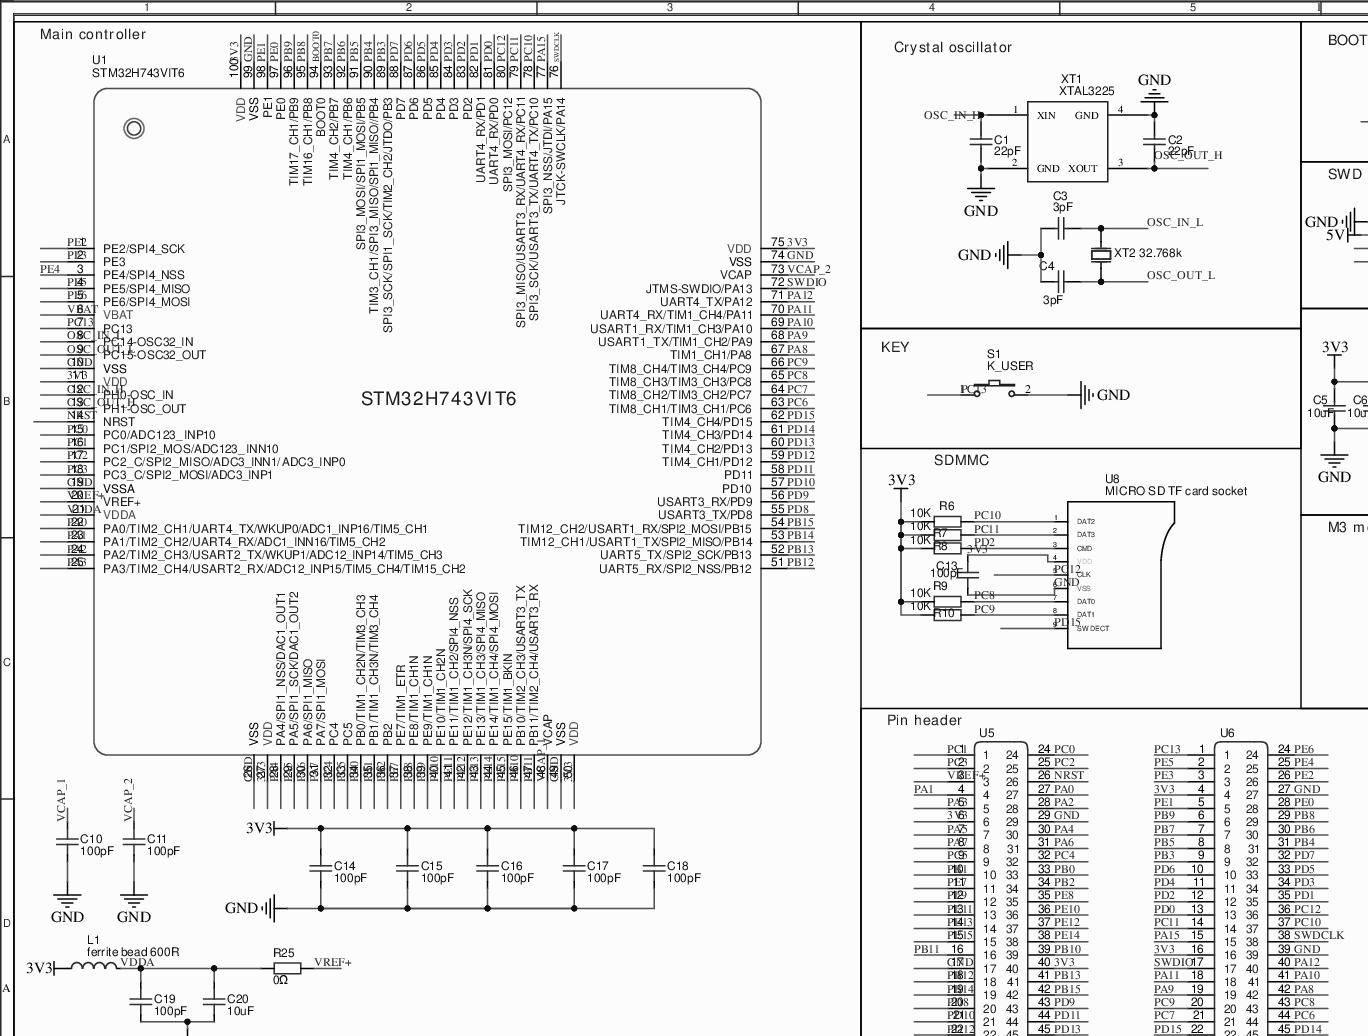
[diagram p0: MISC51975-3.schdoc, top left]
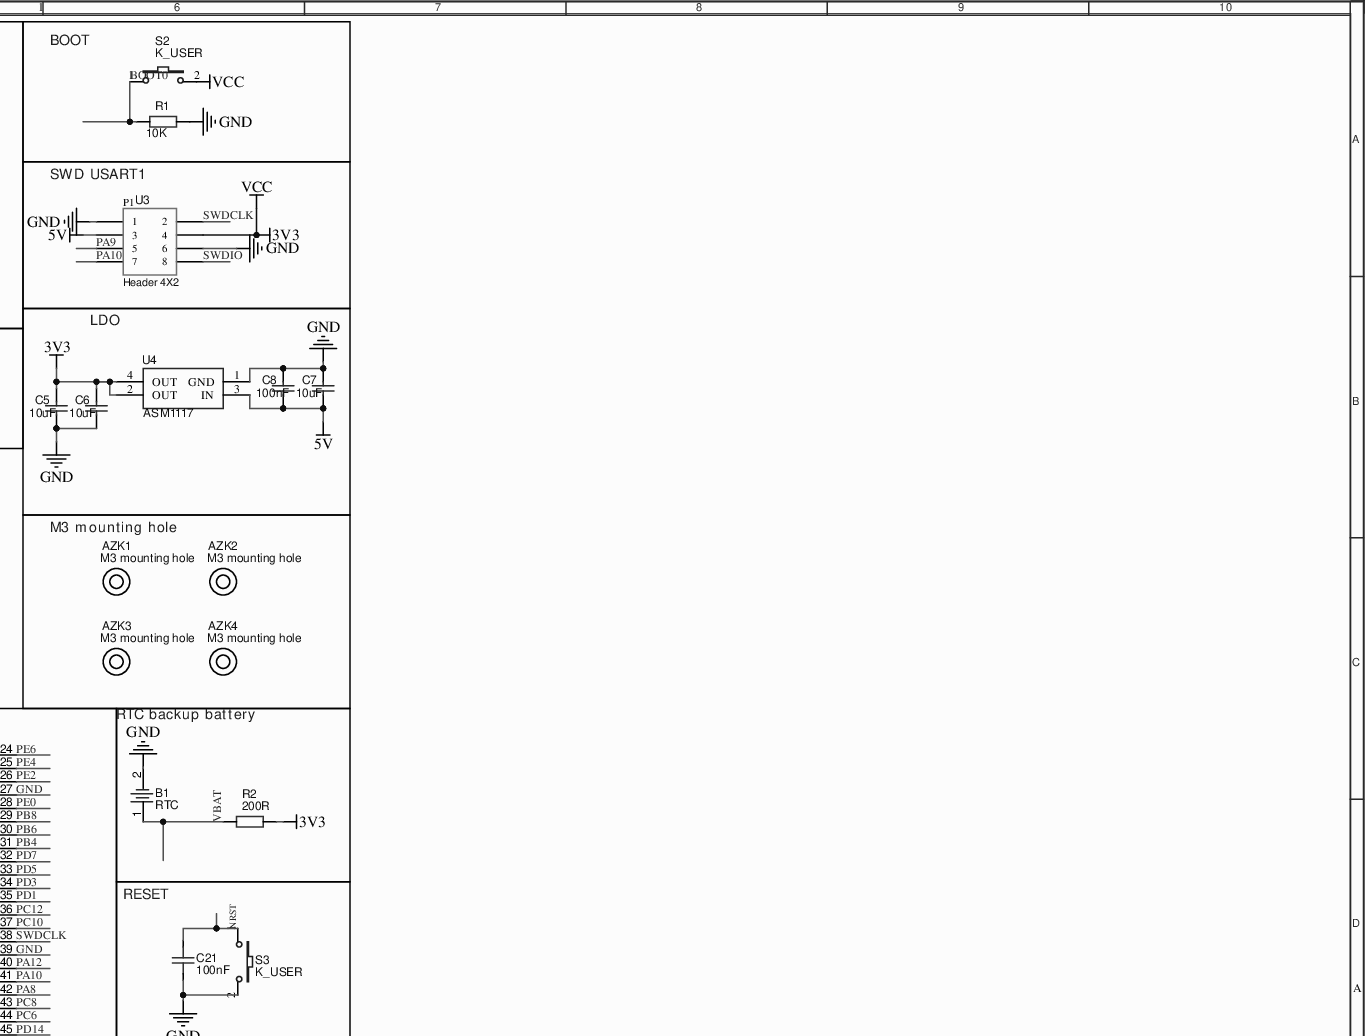
[diagram p1: MISC51975-3.schdoc, top right]
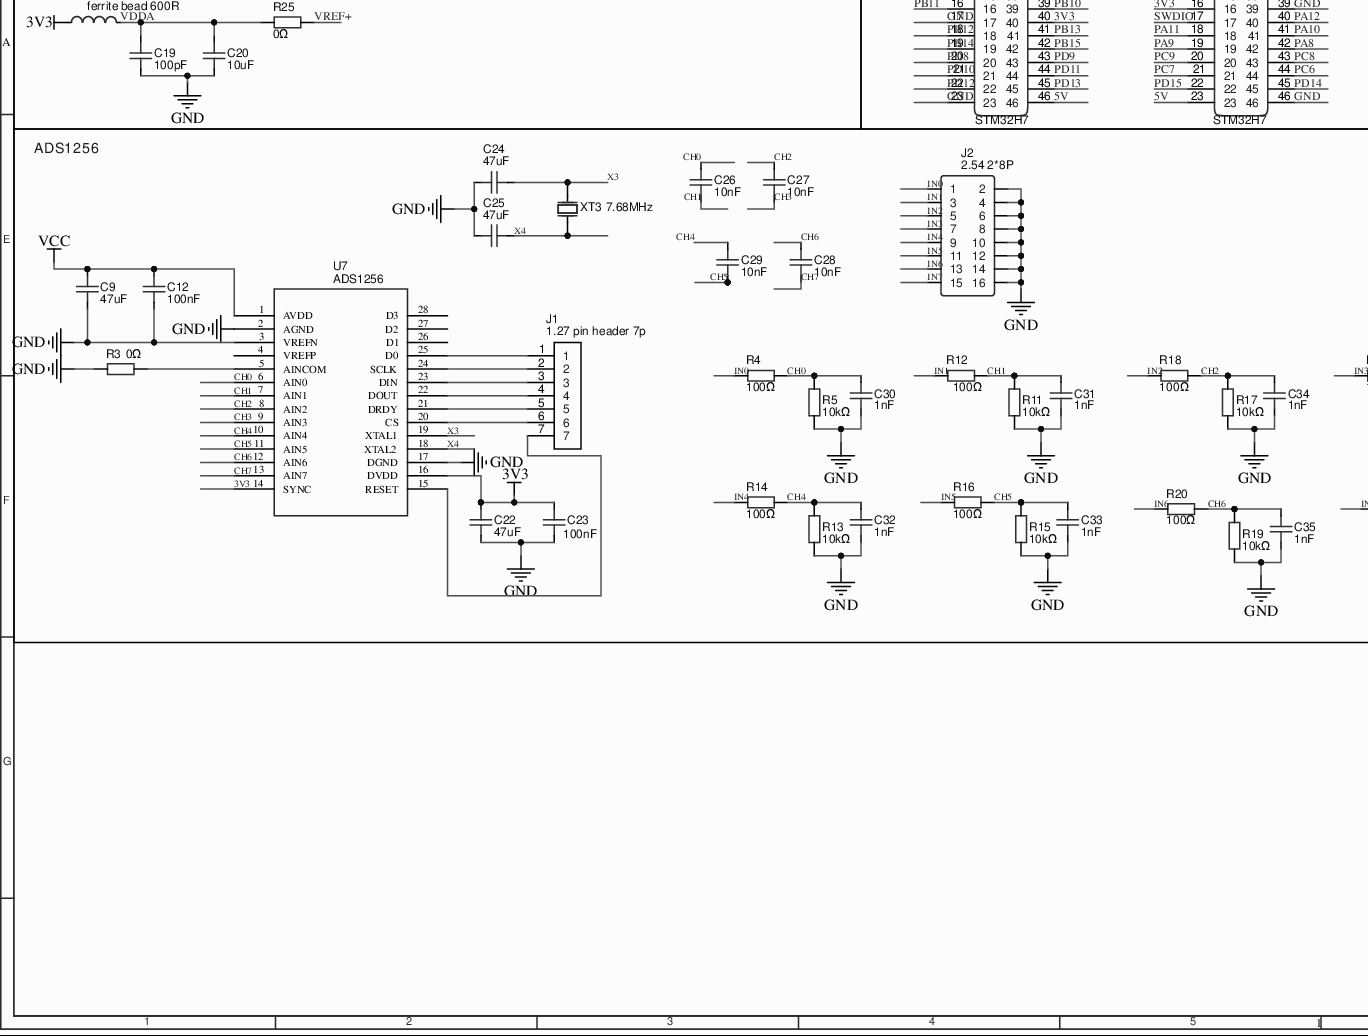
[diagram p2: MISC51975-3.schdoc, bottom left]
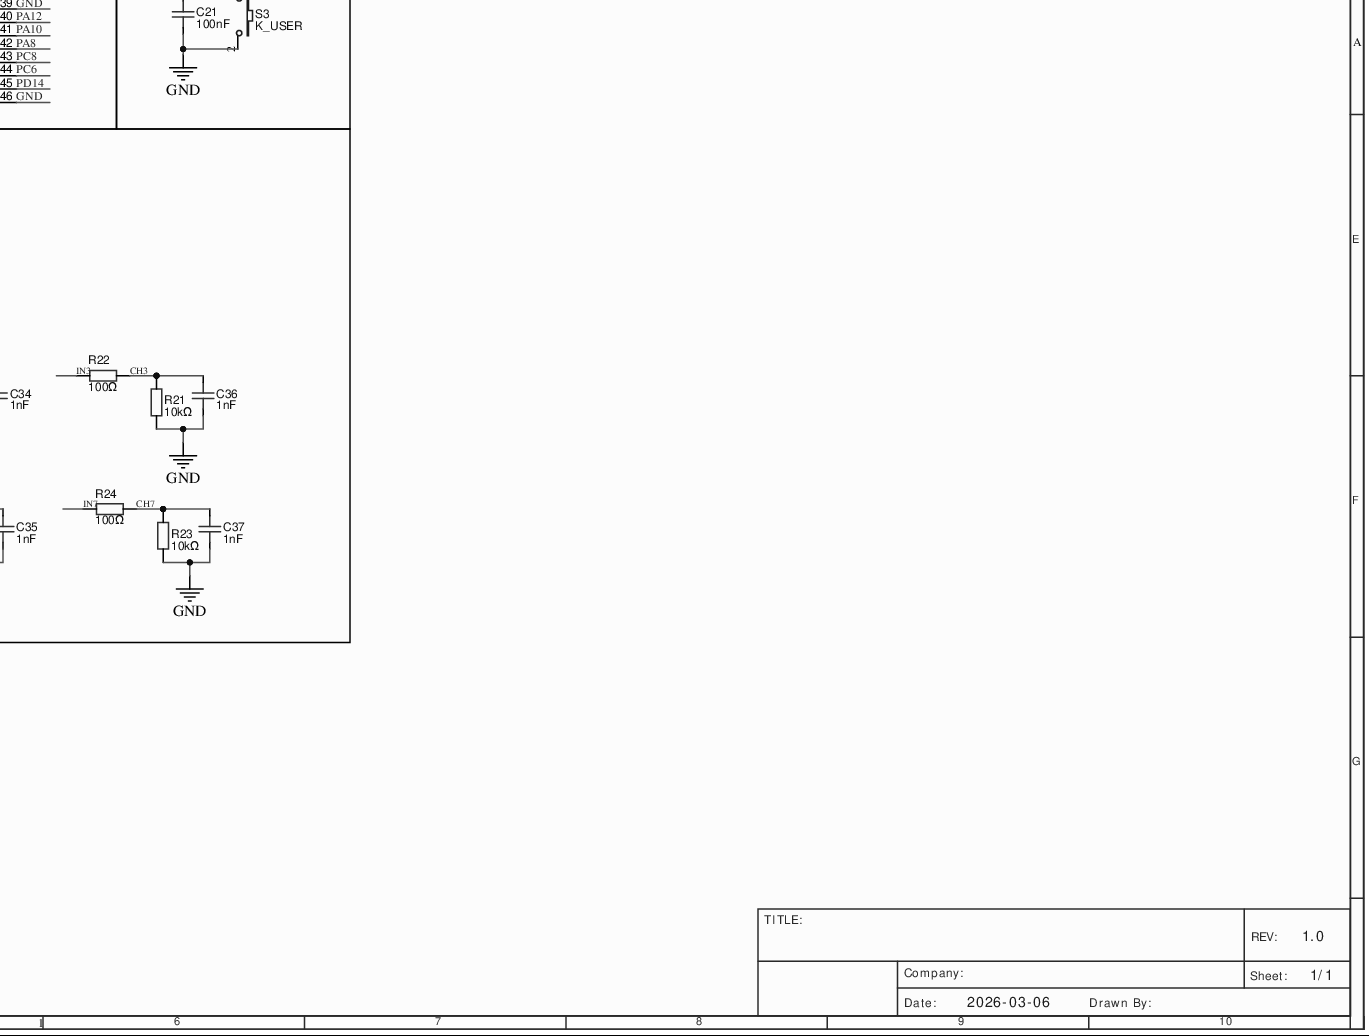
[diagram p3: MISC51975-3.schdoc, bottom right]
# Altium project MISC51975-2.PrjPcb
1 sheet, 83 parts. Net scope: global (net labels, ports and power ports of the same name join across sheets).
Board file: MISC51975.pcbdoc

## Sheet MISC51975-3.schdoc
size 503 x 376 mm; Name: MISC51975; @Project Name: MISC51975; REV: 1.0; Date: 2026-03-06; Sheet: 1/1; Manufacturer Part: ?

### Parts
AZK1  M3 mounting hole  [M3安装孔(非金属化)]
AZK2  M3 mounting hole  [M3安装孔(非金属化)]
AZK3  M3 mounting hole  [M3安装孔(非金属化)]
AZK4  M3 mounting hole  [M3安装孔(非金属化)]
B1  RTC  [焊盘引出RTC]
C1  22pF  [C0402]
C2  22pF  [C0402]
C3  3pF  [C0402]
C4  3pF  [C0402]
C5  10uF  [C0402]
C6  10uF  [C0402]
C7  10uF  [C0402]
C8  100nF  [C0402]
C9  47uF  [C0402]
C10  100pF  [C0402]
C11  100pF  [C0402]
C12  100nF  [C0402]
C13  100pF  [C0402]
C14  100pF  [C0402]
C15  100pF  [C0402]
C16  100pF  [C0402]
C17  100pF  [C0402]
C18  100pF  [C0402]
C19  100pF  [C0402]
C20  10uF  [C0402]
C21  100nF  [C0402]
C22  47uF  [C0402]
C23  100nF  [C0402]
C24  47uF  [C0402]
C25  47uF  [C0402]
C26  10nF  [C0402]
C27  10nF  [C0402]
C28  10nF  [C0402]
C29  10nF  [C0402]
C30  1nF  [C0402]
C31  1nF  [C0402]
C32  1nF  [C0402]
C33  1nF  [C0402]
C34  1nF  [C0402]
C35  1nF  [C0402]
C36  1nF  [C0402]
C37  1nF  [C0402]
J1  1.27 pin header 7p  [1.27排针7P]
J2  2.54 2*8P  [HDR-TH_16P-P2.54-V-R2-C8-S2.54]
L1  ferrite bead 600R  [L0402]
R1  10K  [贴片电阻0402封装]
R2  200R  [贴片电阻0402封装]
R3  0Ω  [贴片电阻0402封装]
R4  100Ω  [贴片电阻0402封装]
R5  10kΩ  [贴片电阻0402封装]
R6  10K  [贴片电阻0402封装]
R7  10K  [贴片电阻0402封装]
R8  10K  [贴片电阻0402封装]
R9  10K  [贴片电阻0402封装]
R10  10K  [贴片电阻0402封装]
R11  10kΩ  [贴片电阻0402封装]
R12  100Ω  [贴片电阻0402封装]
R13  10kΩ  [贴片电阻0402封装]
R14  100Ω  [贴片电阻0402封装]
R15  10kΩ  [贴片电阻0402封装]
R16  100Ω  [贴片电阻0402封装]
R17  10kΩ  [贴片电阻0402封装]
R18  100Ω  [贴片电阻0402封装]
R19  10kΩ  [贴片电阻0402封装]
R20  100Ω  [贴片电阻0402封装]
R21  10kΩ  [贴片电阻0402封装]
R22  100Ω  [贴片电阻0402封装]
R23  10kΩ  [贴片电阻0402封装]
R24  100Ω  [贴片电阻0402封装]
R25  0Ω  [贴片电阻0402封装]
S1  K_USER  [按键开关4.5]
S2  K_USER  [按键开关4.5]
S3  K_USER  [按键开关4.5]
U1  STM32H743VIT6  [STM32H743VIT6]
U3  HDR_2*4P  [HDR_2*4P]  (value not drawn)
U4  ASM1117  [AMS1117-SOT-223]
U5  STM32H7  [2*23]
U6  STM32H7  [2*23]
U7  ADS1256  [SSOP-28_L10.2-W5.3-P0.65-LS7.8-BL]
U8  MICRO SD TF card socket  [MICRO SD TF卡座]
XT1  XTAL3225  [XTAL3225]
XT2  32.768k  [SMD-2012_2P]
XT3  7.68MHz  [SMD-2012_2P]

### Blocks framed on the sheet
Main controller: C10 C11 C14-C20 L1 R25 U1
Crystal oscillator: C1-C4 XT1 XT2
BOOT: R1 S2
SWD USART1: U3
KEY: S1
LDO: C5-C8 U4
M3 mounting hole: AZK1-AZK4
Pin header: U5 U6
RTC backup battery: B1 R2
RESET: C21 S3
ADS1256: C9 C12 C22-C37 J1 J2 R3-R5 R11-R24 U7 XT3

### Nets
3V3: C5.2 C6.2 C9.2 C12.2 C13.2 C14.2 C15.2 C16.2 C17.2 C18.2 C22.2 C23.2 L1.1 R2.1 R6.1 R7.1 R8.1 R9.1 R10.1 S2.2 U1.11(VDD) U1.27(VDD) U1.50(VDD) U1.75(VDD) U1.100(VDD) U3.4 U4.2(OUT) U4.4(OUT) U5.6 U5.40 U6.4 U6.16 U7.1(AVDD) U7.14(SYNC) U7.16(DVDD) U8.4(VDD)  [also labelled VCC]
5V: C7.1 C8.1 U3.3 U4.3(IN) U5.46 U6.23
GND: B1.2 C1.1 C2.2 C3.2 C4.2 C5.1 C6.1 C7.2 C8.2 C9.1 C10.1 C11.1 C12.1 C13.1 C14.1 C15.1 C16.1 C17.1 C18.1 C19.1 C20.1 C21.1 C22.1 C23.1 C24.2 C25.2 C30.2 C31.2 C32.2 C33.2 C34.2 C35.2 C36.2 C37.2 J2.2 J2.4 J2.6 J2.8 J2.10 J2.12 J2.14 J2.16 R1.2 R3.1 R5.1 R11.1 R13.1 R15.1 R17.1 R19.1 R21.1 R23.1 S1.2 S3.2 U1.10(VSS) U1.19(VSSA) U1.26(VSS) U1.49(VSS) U1.74(VSS) U1.99(VSS) U3.1 U3.6 U4.1(GND) U5.17 U5.23 U5.29 U6.27 U6.39 U6.46 U7.2(AGND) U7.3(VREFN) U7.17(DGND) U8.6(VSS) XT1.2(GND) XT1.4(GND)
BOOT0: R1.1 S2.1 U1.94(BOOT0)
CH0: C26.1 C30.1 R4.2 R5.2 U7.6(AIN0)
CH1: C26.2 C31.1 R11.2 R12.2 U7.7(AIN1)
CH2: C27.1 C34.1 R17.2 R18.2 U7.8(AIN2)
CH3: C27.2 C36.1 R21.2 R22.2 U7.9(AIN3)
CH4: C29.1 C32.1 R13.2 R14.2 U7.10(AIN4)
CH5: C29.2 C33.1 R15.2 R16.2 U7.11(AIN5)
CH6: C28.1 C35.1 R19.2 R20.2 U7.12(AIN6)
CH7: C28.2 C37.1 R23.2 R24.2 U7.13(AIN7)
IN0: J2.1 R4.1
IN1: J2.3 R12.1
IN2: J2.5 R18.1
IN3: J2.7 R22.1
IN4: J2.9 R14.1
IN5: J2.11 R16.1
IN6: J2.13 R20.1
IN7: J2.15 R24.1
NRST: C21.2 S3.1 U1.14(NRST) U5.26
OSC_IN_H: C1.2 U1.12(PH0-OSC_IN) XT1.1(XIN)
OSC_IN_L: C3.1 U1.8(PC14-OSC32_IN) XT2.1(OSC1)
OSC_OUT_H: C2.1 U1.13(PH1-OSC_OUT) XT1.3(XOUT)
OSC_OUT_L: C4.1 U1.9(PC15-OSC32_OUT) XT2.2(OSC2)
PA0: U1.22(PA0/TIM2_CH1/UART4_TX/WKUP0/ADC1_INP16/TIM5_CH1) U5.27
PA1: U1.23(PA1/TIM2_CH2/UART4_RX/ADC1_INN16/TIM5_CH2) U5.4
PA2: U1.24(PA2/TIM2_CH3/USART2_TX/WKUP1/ADC12_INP14/TIM5_CH3) U5.28
PA3: U1.25(PA3/TIM2_CH4/USART2_RX/ADC12_INP15/TIM5_CH4/TIM15_CH2) U5.5
PA4: U1.28(PA4/SPI1_NSS/DAC1_OUT1) U5.30
PA5: U1.29(PA5/SPI1_SCK/DAC1_OUT2) U5.7
PA6: U1.30(PA6/SPI1_MISO) U5.31
PA7: U1.31(PA7/SPI1_MOSI) U5.8
PA8: U1.67(TIM1_CH1/PA8) U6.42
PA9: U1.68(USART1_TX/TIM1_CH2/PA9) U3.5 U6.19
PA10: U1.69(USART1_RX/TIM1_CH3/PA10) U3.7 U6.41
PA11: U1.70(UART4_RX/TIM1_CH4/PA11) U6.18
PA12: U1.71(UART4_TX/PA12) U6.40
PA15: U1.77(SPI3_NSS/JTDI/PA15) U6.15
PB0: U1.34(PB0/TIM1_CH2N/TIM3_CH3) U5.33
PB1: U1.35(PB1/TIM1_CH3N/TIM3_CH4) U5.10
PB2: U1.36(PB2) U5.34
PB3: U1.89(SPI3_SCK/SPI1_SCK/TIM2_CH2/JTDO/PB3) U6.9
PB4: U1.90(TIM3_CH1/SPI3_MISO/SPI1_MISO//PB4) U6.31
PB5: U1.91(SPI3_MOSI/SPI1_MOSI/PB5) U6.8
PB6: U1.92(TIM4_CH1/PB6) U6.30
PB7: U1.93(TIM4_CH2/PB7) U6.7
PB8: U1.95(TIM16_CH1/PB8) U6.29
PB9: U1.96(TIM17_CH1/PB9) U6.6
PB10: U1.46(PB10/TIM2_CH3/USART3_TX) U5.39
PB11: U1.47(PB11/TIM2_CH4/USART3_RX) U5.16
PB12: U1.51(UART5_RX/SPI2_NSS/PB12) U5.18
PB13: U1.52(UART5_TX/SPI2_SCK/PB13) U5.41
PB14: U1.53(TIM12_CH1/USART1_TX/SPI2_MISO/PB14) U5.19
PB15: U1.54(TIM12_CH2/USART1_RX/SPI2_MOSI/PB15) U5.42
PC0: U1.15(PC0/ADC123__INP10) U5.24
PC1: U1.16(PC1/SPI2_MOS/ADC123__INN10) U5.1
PC2: U1.17(PC2_C/SPI2_MISO/ADC3_INN1/_ADC3_INP0) U5.25
PC3: U1.18(PC3_C/SPI2_MOSI/ADC3_INP1) U5.2
PC4: U1.32(PC4) U5.32
PC5: U1.33(PC5) U5.9
PC6: U1.63(TIM8_CH1/TIM3_CH1/PC6) U6.44
PC7: U1.64(TIM8_CH2/TIM3_CH2/PC7) U6.21
PC8: R9.2 U1.65(TIM8_CH3/TIM3_CH3/PC8) U6.43 U8.7(DAT0)
PC9: R10.2 U1.66(TIM8_CH4/TIM3_CH4/PC9) U6.20 U8.8(DAT1)
PC10: R6.2 U1.78(SPI3_SCK/USART3_TX/UART4_TX/PC10) U6.37 U8.1(DAT2)
PC11: R7.2 U1.79(SPI3_MISO/USART3_RX/UART4_RX/PC11) U6.14 U8.2(DAT3)
PC12: U1.80(SPI3_MOSI/PC12) U6.36 U8.5(CLK)
PC13: S1.1 U1.7(PC13) U6.1
PD0: U1.81(UART4_RX/PD0) U6.13
PD1: U1.82(UART4_RX/PD1) U6.35
PD2: R8.2 U1.83(PD2) U6.12 U8.3(CMD)
PD3: U1.84(PD3) U6.34
PD4: U1.85(PD4) U6.11
PD5: U1.86(PD5) U6.33
PD6: U1.87(PD6) U6.10
PD7: U1.88(PD7) U6.32
PD8: U1.55(USART3_TX/PD8) U5.20
PD9: U1.56(USART3_RX/PD9) U5.43
PD10: U1.57(PD10) U5.21
PD11: U1.58(PD11) U5.44
PD12: U1.59(TIM4_CH1/PD12) U5.22
PD13: U1.60(TIM4_CH2/PD13) U5.45
PD14: U1.61(TIM4_CH3/PD14) U6.45
PD15: U1.62(TIM4_CH4/PD15) U6.22 U8.9(SW_DECT)
PE0: U1.97(PE0) U6.28
PE1: U1.98(PE1) U6.5
PE2: U1.1(PE2/SPI4_SCK) U6.26
PE3: U1.2(PE3) U6.3
PE4: U1.3(PE4/SPI4_NSS) U6.25
PE5: U1.4(PE5/SPI4_MISO) U6.2
PE6: U1.5(PE6/SPI4_MOSI) U6.24
PE7: U1.37(PE7/TIM1_ETR) U5.11
PE8: U1.38(PE8/TIM1_CH1N) U5.35
PE9: U1.39(PE9/TIM1_CH1N) U5.12
PE10: U1.40(PE10/TIM1_CH2N) U5.36
PE11: U1.41(PE11/TIM1_CH2/SPI4_NSS) U5.13
PE12: U1.42(PE12/TIM1_CH3N/SPI4_SCK) U5.37
PE13: U1.43(PE13/TIM1_CH3/SPI4_MISO) U5.14
PE14: U1.44(PE14/TIM1_CH4/SPI4_MOSI) U5.38
PE15: U1.45(PE15/TIM1_BKIN) U5.15
SWDCLK: U1.76(JTCK-SWCLK/PA14) U3.2 U6.38
SWDIO: U1.72(JTMS-SWDIO/PA13) U3.8 U6.17
VBAT: B1.1 R2.2 U1.6(VBAT)
VCAP_1: C10.2 U1.48(VCAP)
VCAP_2: C11.2 U1.73(VCAP)
VDDA: C19.2 C20.2 L1.2 R25.1 U1.21(VDDA)
VREF+: R25.2 U1.20(VREF+) U5.3
X3: C24.1 U7.19(XTAL1) XT3.1(OSC1)
X4: C25.1 U7.18(XTAL2) XT3.2(OSC2)
NetJ1_1: J1.1 U7.25(D0)
NetJ1_2: J1.2 U7.24(SCLK)
NetJ1_3: J1.3 U7.23(DIN)
NetJ1_4: J1.4 U7.22(DOUT)
NetJ1_5: J1.5 U7.21(DRDY)
NetJ1_6: J1.6 U7.20(CS)
NetJ1_7: J1.7 U7.15(RESET)
NetR3_2: R3.2 U7.5(AINCOM)

Not connected (* = marked no-connect by the designer): U7 4(VREFP)* 26(D1)* 27(D2)* 28(D3)*

### Notes on the sheet
- SDMMC
- 1
- 2
- 3
- 4
- 5
- 6
- 7
- 8
- 9
- 10
- A
- B
- C
- D
- E
- F
- G
- TITLE:
- Company:
- Sheet:
- REV:
- 1.0
- 1/1
- Date:
- 2026-03-06
- Drawn By:

### Library data of the parts
AZK1 = M3安装孔: Convert to PCB: yes; Add into BOM: no; UniqueId: gge2d938f74b51f9b54; Device: M3 mounting hole; SymbolName: M3 mounting hole; FootprintName: M3 mounting hole (non-plated)
AZK2 = M3安装孔: Convert to PCB: yes; Add into BOM: no; UniqueId: gge66d1f239ac2c5538; Device: M3 mounting hole; SymbolName: M3 mounting hole; FootprintName: M3 mounting hole (non-plated)
AZK3 = M3安装孔: Convert to PCB: yes; Add into BOM: no; UniqueId: gge752a5f65646d66a6; Device: M3 mounting hole; SymbolName: M3 mounting hole; FootprintName: M3 mounting hole (non-plated)
AZK4 = M3安装孔: Convert to PCB: yes; Add into BOM: no; UniqueId: gge6f756c0247ec58fb; Device: M3 mounting hole; SymbolName: M3 mounting hole; FootprintName: M3 mounting hole (non-plated)
B1 = RTC: Convert to PCB: yes; UniqueId: gge9c6e9f6a6062b857; OriginModelName: BAT-SMD_CR1220-2; ModelTransform: 777.81069,586.46209,0,180,0,0,-46.024,-3.307,-31.496; Device: RTC; Add into BOM: yes; SymbolName: RTC; FootprintName: Pad lead-out RTC
C1 = 0402CG220J500NT: Manufacturer: FH(风华); Convert to PCB: yes; UniqueId: ggeb8d6d3f9e94ab257; OriginModelName: C0402_L1.0-W0.5-H0.5; ModelTransform: 39.37,19.685,0,0,0,0,0,0.001,0; Device: 0402CG220J500NT; Supplier: LCSC; Manufacturer Part: 0402CG220J500NT; Supplier Part: C1555; JLCPCB Part Class: Basic Part; Add into BOM: yes; SymbolName: 22pF; FootprintName: C0402
C2 = 0402CG220J500NT: Manufacturer: FH(风华); Convert to PCB: yes; UniqueId: gge5bf67a0cc8ec0b42; OriginModelName: C0402_L1.0-W0.5-H0.5; ModelTransform: 39.37,19.685,0,0,0,0,0,0.001,0; Device: 0402CG220J500NT; Supplier: LCSC; Manufacturer Part: 0402CG220J500NT; Supplier Part: C1555; JLCPCB Part Class: Basic Part; Add into BOM: yes; SymbolName: 22pF; FootprintName: C0402
C3 = 0402CG220J500NT: Manufacturer: FH(风华); Convert to PCB: yes; UniqueId: gge026c9d84113bc248; OriginModelName: C0402_L1.0-W0.5-H0.5; ModelTransform: 39.37,19.685,0,0,0,0,0,0.001,0; Device: 0402CG220J500NT; Supplier: LCSC; Manufacturer Part: 0402CG220J500NT; Supplier Part: C1555; JLCPCB Part Class: Basic Part; Add into BOM: yes; SymbolName: 3pF; FootprintName: C0402
C4 = 0402CG220J500NT: Manufacturer: FH(风华); Convert to PCB: yes; UniqueId: ggeb5b0492ef2ec8ab9; OriginModelName: C0402_L1.0-W0.5-H0.5; ModelTransform: 39.37,19.685,0,0,0,0,0,0.001,0; Device: 0402CG220J500NT; Supplier: LCSC; Manufacturer Part: 0402CG220J500NT; Supplier Part: C1555; JLCPCB Part Class: Basic Part; Add into BOM: yes; SymbolName: 3pF; FootprintName: C0402
C5 = 0402CG220J500NT: Manufacturer: FH(风华); Convert to PCB: yes; UniqueId: gge2a57da8ad470d0b7; OriginModelName: C0402_L1.0-W0.5-H0.5; ModelTransform: 39.37,19.685,0,0,0,0,0,0.001,0; Device: 0402CG220J500NT; Supplier: LCSC; Manufacturer Part: 0402CG220J500NT; Supplier Part: C1555; JLCPCB Part Class: Basic Part; Add into BOM: yes; SymbolName: 10uF; FootprintName: C0402
C6 = 0402CG220J500NT: Manufacturer: FH(风华); Convert to PCB: yes; UniqueId: gge47b3f01545f1c626; OriginModelName: C0402_L1.0-W0.5-H0.5; ModelTransform: 39.37,19.685,0,0,0,0,0,0.001,0; Device: 0402CG220J500NT; Supplier: LCSC; Manufacturer Part: 0402CG220J500NT; Supplier Part: C1555; JLCPCB Part Class: Basic Part; Add into BOM: yes; SymbolName: 10uF; FootprintName: C0402
C7 = 0402CG220J500NT: Manufacturer: FH(风华); Convert to PCB: yes; UniqueId: gge634d3278784ec25c; OriginModelName: C0402_L1.0-W0.5-H0.5; ModelTransform: 39.37,19.685,0,0,0,0,0,0.001,0; Device: 0402CG220J500NT; Supplier: LCSC; Manufacturer Part: 0402CG220J500NT; Supplier Part: C1555; JLCPCB Part Class: Basic Part; Add into BOM: yes; SymbolName: 10uF; FootprintName: C0402
C8 = 0402CG220J500NT: Manufacturer: FH(风华); Convert to PCB: yes; UniqueId: gged471d91c49ba018e; OriginModelName: C0402_L1.0-W0.5-H0.5; ModelTransform: 39.37,19.685,0,0,0,0,0,0.001,0; Device: 0402CG220J500NT; Supplier: LCSC; Manufacturer Part: 0402CG220J500NT; Supplier Part: C1555; JLCPCB Part Class: Basic Part; Add into BOM: yes; SymbolName: 100nF; FootprintName: C0402
C9 = C1005CH2A101K050BA: Manufacturer: TDK; Convert to PCB: yes; UniqueId: gge416e2407aa7b353c; OriginModelName: C0402_L1.0-W0.5-H0.5; ModelTransform: 39.37,19.685,0,0,0,0,0,0.001,0; Device: C1005CH2A101K050BA; Manufacturer Part: C1005CH2A101K050BA; Add into BOM: yes; SymbolName: 47uF; FootprintName: C0402
C10 = C1005CH2A101K050BA: Manufacturer: TDK; Convert to PCB: yes; UniqueId: ggeefce2936f74b20d4; OriginModelName: C0402_L1.0-W0.5-H0.5; ModelTransform: 39.37,19.685,0,0,0,0,0,0.001,0; Device: C1005CH2A101K050BA; Manufacturer Part: C1005CH2A101K050BA; Add into BOM: yes; SymbolName: 100pF; FootprintName: C0402
C11 = C1005CH2A101K050BA: Manufacturer: TDK; Convert to PCB: yes; UniqueId: gge25dcf3aaa99ada2c; OriginModelName: C0402_L1.0-W0.5-H0.5; ModelTransform: 39.37,19.685,0,0,0,0,0,0.001,0; Device: C1005CH2A101K050BA; Manufacturer Part: C1005CH2A101K050BA; Add into BOM: yes; SymbolName: 100pF; FootprintName: C0402
C12 = C1005CH2A101K050BA: Manufacturer: TDK; Convert to PCB: yes; UniqueId: gge2a0c766e1205cd8b; OriginModelName: C0402_L1.0-W0.5-H0.5; ModelTransform: 39.37,19.685,0,0,0,0,0,0.001,0; Device: C1005CH2A101K050BA; Manufacturer Part: C1005CH2A101K050BA; Add into BOM: yes; SymbolName: 100nF; FootprintName: C0402; Supplier: LCSC; SupplierPart: C1555; JLCPCB Part Class: Basic Part
C13 = C1005CH2A101K050BA: Manufacturer: TDK; Convert to PCB: yes; UniqueId: gge48d7b5d22e7f241c; OriginModelName: C0402_L1.0-W0.5-H0.5; ModelTransform: 39.37,19.685,0,0,0,0,0,0.001,0; Device: C1005CH2A101K050BA; Manufacturer Part: C1005CH2A101K050BA; Add into BOM: yes; SymbolName: 100pF; FootprintName: C0402
C14 = C1005CH2A101K050BA: Manufacturer: TDK; Convert to PCB: yes; UniqueId: gged72f2bf00148525f; OriginModelName: C0402_L1.0-W0.5-H0.5; ModelTransform: 39.37,19.685,0,0,0,0,0,0.001,0; Device: C1005CH2A101K050BA; Manufacturer Part: C1005CH2A101K050BA; Add into BOM: yes; SymbolName: 100pF; FootprintName: C0402
C15 = C1005CH2A101K050BA: Manufacturer: TDK; Convert to PCB: yes; UniqueId: gge454870d93914dfff; OriginModelName: C0402_L1.0-W0.5-H0.5; ModelTransform: 39.37,19.685,0,0,0,0,0,0.001,0; Device: C1005CH2A101K050BA; Manufacturer Part: C1005CH2A101K050BA; Add into BOM: yes; SymbolName: 100pF; FootprintName: C0402
C16 = C1005CH2A101K050BA: Manufacturer: TDK; Convert to PCB: yes; UniqueId: gge947e8dec318f4aa3; OriginModelName: C0402_L1.0-W0.5-H0.5; ModelTransform: 39.37,19.685,0,0,0,0,0,0.001,0; Device: C1005CH2A101K050BA; Manufacturer Part: C1005CH2A101K050BA; Add into BOM: yes; SymbolName: 100pF; FootprintName: C0402
C17 = C1005CH2A101K050BA: Manufacturer: TDK; Convert to PCB: yes; UniqueId: gge4df29904f9385efd; OriginModelName: C0402_L1.0-W0.5-H0.5; ModelTransform: 39.37,19.685,0,0,0,0,0,0.001,0; Device: C1005CH2A101K050BA; Manufacturer Part: C1005CH2A101K050BA; Add into BOM: yes; SymbolName: 100pF; FootprintName: C0402
C18 = C1005CH2A101K050BA: Manufacturer: TDK; Convert to PCB: yes; UniqueId: gge28e10968a2ff1b2b; OriginModelName: C0402_L1.0-W0.5-H0.5; ModelTransform: 39.37,19.685,0,0,0,0,0,0.001,0; Device: C1005CH2A101K050BA; Manufacturer Part: C1005CH2A101K050BA; Add into BOM: yes; SymbolName: 100pF; FootprintName: C0402
C19 = C1005CH2A101K050BA: Manufacturer: TDK; Convert to PCB: yes; UniqueId: gge9cde31d946d041c6; OriginModelName: C0402_L1.0-W0.5-H0.5; ModelTransform: 39.37,19.685,0,0,0,0,0,0.001,0; Device: C1005CH2A101K050BA; Manufacturer Part: C1005CH2A101K050BA; Add into BOM: yes; SymbolName: 100pF; FootprintName: C0402
C20 = C1005CH2A101K050BA: Manufacturer: TDK; Convert to PCB: yes; UniqueId: ggeacee7ace2b0c3443; OriginModelName: C0402_L1.0-W0.5-H0.5; ModelTransform: 39.37,19.685,0,0,0,0,0,0.001,0; Device: C1005CH2A101K050BA; Manufacturer Part: C1005CH2A101K050BA; Add into BOM: yes; SymbolName: 10uF; FootprintName: C0402; Supplier: LCSC; SupplierPart: C1555; JLCPCB Part Class: Basic Part
C21 = C1005CH2A101K050BA: Manufacturer: TDK; Convert to PCB: yes; UniqueId: gge8e3bef2e6c4db5e5; OriginModelName: C0402_L1.0-W0.5-H0.5; ModelTransform: 39.37,19.685,0,0,0,0,0,0.001,0; Device: C1005CH2A101K050BA; Manufacturer Part: C1005CH2A101K050BA; Add into BOM: yes; SymbolName: 100nF; FootprintName: C0402; Supplier: LCSC; SupplierPart: C1555; JLCPCB Part Class: Basic Part
C22 = C1005CH2A101K050BA: Manufacturer: TDK; Convert to PCB: yes; UniqueId: ggef2c99a208792f57a; OriginModelName: C0402_L1.0-W0.5-H0.5; ModelTransform: 39.37,19.685,0,0,0,0,0,0.001,0; Device: C1005CH2A101K050BA; Manufacturer Part: C1005CH2A101K050BA; Add into BOM: yes; SymbolName: 47uF; FootprintName: C0402
C23 = C1005CH2A101K050BA: Manufacturer: TDK; Convert to PCB: yes; UniqueId: gge8a1da77499b18a1b; OriginModelName: C0402_L1.0-W0.5-H0.5; ModelTransform: 39.37,19.685,0,0,0,0,0,0.001,0; Device: C1005CH2A101K050BA; Manufacturer Part: C1005CH2A101K050BA; Add into BOM: yes; SymbolName: 100nF; FootprintName: C0402; Supplier: LCSC; SupplierPart: C1555; JLCPCB Part Class: Basic Part
C24 = C1005CH2A101K050BA: Manufacturer: TDK; Convert to PCB: yes; UniqueId: gge5964156e8627b443; OriginModelName: C0402_L1.0-W0.5-H0.5; ModelTransform: 39.37,19.685,0,0,0,0,0,0.001,0; Device: C1005CH2A101K050BA; Manufacturer Part: C1005CH2A101K050BA; Add into BOM: yes; SymbolName: 47uF; FootprintName: C0402
C25 = C1005CH2A101K050BA: Manufacturer: TDK; Convert to PCB: yes; UniqueId: ggea1632ea0a53482c7; OriginModelName: C0402_L1.0-W0.5-H0.5; ModelTransform: 39.37,19.685,0,0,0,0,0,0.001,0; Device: C1005CH2A101K050BA; Manufacturer Part: C1005CH2A101K050BA; Add into BOM: yes; SymbolName: 47uF; FootprintName: C0402
C26 = C1005CH2A101K050BA: Manufacturer: TDK; Convert to PCB: yes; UniqueId: gge335505e1f9403f52; OriginModelName: C0402_L1.0-W0.5-H0.5; ModelTransform: 39.37,19.685,0,0,0,0,0,0.001,0; Device: C1005CH2A101K050BA; Manufacturer Part: C1005CH2A101K050BA; Add into BOM: yes; SymbolName: 10nF; FootprintName: C0402
C27 = C1005CH2A101K050BA: Manufacturer: TDK; Convert to PCB: yes; UniqueId: gge35a144984d2c3980; OriginModelName: C0402_L1.0-W0.5-H0.5; ModelTransform: 39.37,19.685,0,0,0,0,0,0.001,0; Device: C1005CH2A101K050BA; Manufacturer Part: C1005CH2A101K050BA; Add into BOM: yes; SymbolName: 10nF; FootprintName: C0402
C28 = C1005CH2A101K050BA: Manufacturer: TDK; Convert to PCB: yes; UniqueId: gge50e500b25d1be4b6; OriginModelName: C0402_L1.0-W0.5-H0.5; ModelTransform: 39.37,19.685,0,0,0,0,0,0.001,0; Device: C1005CH2A101K050BA; Manufacturer Part: C1005CH2A101K050BA; Add into BOM: yes; SymbolName: 10nF; FootprintName: C0402
C29 = C1005CH2A101K050BA: Manufacturer: TDK; Convert to PCB: yes; UniqueId: gge010c584659bff661; OriginModelName: C0402_L1.0-W0.5-H0.5; ModelTransform: 39.37,19.685,0,0,0,0,0,0.001,0; Device: C1005CH2A101K050BA; Manufacturer Part: C1005CH2A101K050BA; Add into BOM: yes; SymbolName: 10nF; FootprintName: C0402
C30 = C1005CH2A101K050BA: Manufacturer: TDK; Convert to PCB: yes; UniqueId: gge53ed05ade17cbd9b; OriginModelName: C0402_L1.0-W0.5-H0.5; ModelTransform: 39.37,19.685,0,0,0,0,0,0.001,0; Device: C1005CH2A101K050BA; Manufacturer Part: C1005CH2A101K050BA; Add into BOM: yes; SymbolName: 1nF; FootprintName: C0402
C31 = C1005CH2A101K050BA: Manufacturer: TDK; Convert to PCB: yes; UniqueId: ggee5c0126d94065c1b; OriginModelName: C0402_L1.0-W0.5-H0.5; ModelTransform: 39.37,19.685,0,0,0,0,0,0.001,0; Device: C1005CH2A101K050BA; Manufacturer Part: C1005CH2A101K050BA; Add into BOM: yes; SymbolName: 1nF; FootprintName: C0402
C32 = C1005CH2A101K050BA: Manufacturer: TDK; Convert to PCB: yes; UniqueId: ggeebfdc114e9a0ab79; OriginModelName: C0402_L1.0-W0.5-H0.5; ModelTransform: 39.37,19.685,0,0,0,0,0,0.001,0; Device: C1005CH2A101K050BA; Manufacturer Part: C1005CH2A101K050BA; Add into BOM: yes; SymbolName: 1nF; FootprintName: C0402
C33 = C1005CH2A101K050BA: Manufacturer: TDK; Convert to PCB: yes; UniqueId: ggeb72b5da5d762d6af; OriginModelName: C0402_L1.0-W0.5-H0.5; ModelTransform: 39.37,19.685,0,0,0,0,0,0.001,0; Device: C1005CH2A101K050BA; Manufacturer Part: C1005CH2A101K050BA; Add into BOM: yes; SymbolName: 1nF; FootprintName: C0402
C34 = C1005CH2A101K050BA: Manufacturer: TDK; Convert to PCB: yes; UniqueId: ggec653eb8415e46d01; OriginModelName: C0402_L1.0-W0.5-H0.5; ModelTransform: 39.37,19.685,0,0,0,0,0,0.001,0; Device: C1005CH2A101K050BA; Manufacturer Part: C1005CH2A101K050BA; Add into BOM: yes; SymbolName: 1nF; FootprintName: C0402
C35 = C1005CH2A101K050BA: Manufacturer: TDK; Convert to PCB: yes; UniqueId: ggece7a76ce824be026; OriginModelName: C0402_L1.0-W0.5-H0.5; ModelTransform: 39.37,19.685,0,0,0,0,0,0.001,0; Device: C1005CH2A101K050BA; Manufacturer Part: C1005CH2A101K050BA; Add into BOM: yes; SymbolName: 1nF; FootprintName: C0402
C36 = C1005CH2A101K050BA: Manufacturer: TDK; Convert to PCB: yes; UniqueId: gge05a4e1bf05e30a87; OriginModelName: C0402_L1.0-W0.5-H0.5; ModelTransform: 39.37,19.685,0,0,0,0,0,0.001,0; Device: C1005CH2A101K050BA; Manufacturer Part: C1005CH2A101K050BA; Add into BOM: yes; SymbolName: 1nF; FootprintName: C0402
C37 = C1005CH2A101K050BA: Manufacturer: TDK; Convert to PCB: yes; UniqueId: gge23b2269ed92f9486; OriginModelName: C0402_L1.0-W0.5-H0.5; ModelTransform: 39.37,19.685,0,0,0,0,0,0.001,0; Device: C1005CH2A101K050BA; Manufacturer Part: C1005CH2A101K050BA; Add into BOM: yes; SymbolName: 1nF; FootprintName: C0402
J1 = 1.27排针7p: Convert to PCB: yes; UniqueId: ggeac47c2f3a7df920d; Device: 1.27 pin header 7p; Add into BOM: yes; SymbolName: 1.27 pin header 7p; FootprintName: 1.27 pin header 7P
J2 = 2.54mm,2×8Double female header: Manufacturer: BOOMELE; Convert to PCB: yes; UniqueId: ggeaa5d80130c82fba4; OriginModelName: HDR2.54-F-LI-2X8P; ModelTransform: 799.99844,200,0,0,0,0,0,0,-118.11; Device: 2.54mm,2×8Double female header; Supplier: LCSC; Manufacturer Part: 2.54mm,2×8Double female header; image: C30734.jpg; Supplier Part: C30734; Add into BOM: yes; SymbolName: 2.54 2*8P; FootprintName: HDR-TH_16P-P2.54-V-R2-C8-S2.54
L1 = SDCL1005C22NJTDF: Manufacturer: Sunlord; Convert to PCB: yes; UniqueId: ggeb9a1739ff7478abc; OriginModelName: L0402_L1.0-W0.5-H0.5_BEAD; ModelTransform: 39.37,19.685,0,0,0,0,0,0.001,0; Device: SDCL1005C22NJTDF; Supplier: LCSC; Manufacturer Part: SDCL1005C22NJTDF; Supplier Part: C27145; JLCPCB Part Class: Extended Part; Add into BOM: yes; SymbolName: ferrite bead 600R; FootprintName: L0402
R1 = RMC080510K1%N: Manufacturer: Tyohm(幸亚电阻); Resistance (Ohms): ?K; Convert to PCB: yes; UniqueId: gge607ca17142507f3f; OriginModelName: R0402_L1.0-W0.5-H0.5; ModelTransform: 39.37,19.685,0,0,0,0,0,0.001,0; Device: RMC080510K1%N; Supplier: LCSC; Supplier Part: C269742; Manufacturer Part: RMC080510K1%N; JLCPCB Part Class: Extended Part; Add into BOM: yes; SymbolName: 10K; FootprintName: SMD resistor 0402 package
R2 = RMC080510K1%N: Manufacturer: Tyohm(幸亚电阻); Resistance (Ohms): ?K; Convert to PCB: yes; UniqueId: ggec1b409bea39a44f2; OriginModelName: R0402_L1.0-W0.5-H0.5; ModelTransform: 39.37,19.685,0,0,0,0,0,0.001,0; Device: RMC080510K1%N; Supplier: LCSC; Supplier Part: C269742; Manufacturer Part: RMC080510K1%N; JLCPCB Part Class: Extended Part; Add into BOM: yes; SymbolName: 200R; FootprintName: SMD resistor 0402 package
R3 = RMC080510K1%N: Manufacturer: Tyohm(幸亚电阻); Resistance (Ohms): ?K; Convert to PCB: yes; UniqueId: gge3632dfd9d95a716b; OriginModelName: R0402_L1.0-W0.5-H0.5; ModelTransform: 39.37,19.685,0,0,0,0,0,0.001,0; Device: RMC080510K1%N; Supplier: LCSC; Supplier Part: C269742; Manufacturer Part: RMC080510K1%N; JLCPCB Part Class: Extended Part; Add into BOM: yes; SymbolName: 0Ω; FootprintName: SMD resistor 0402 package
R4 = RMC080510K1%N: Manufacturer: Tyohm(幸亚电阻); Resistance (Ohms): ?K; Convert to PCB: yes; UniqueId: gge19dd70609cfd022c; OriginModelName: R0402_L1.0-W0.5-H0.5; ModelTransform: 39.37,19.685,0,0,0,0,0,0.001,0; Device: RMC080510K1%N; Supplier: LCSC; Supplier Part: C269742; Manufacturer Part: RMC080510K1%N; JLCPCB Part Class: Extended Part; Add into BOM: yes; SymbolName: 100Ω; FootprintName: SMD resistor 0402 package
R5 = RMC080510K1%N: Manufacturer: Tyohm(幸亚电阻); Resistance (Ohms): ?K; Convert to PCB: yes; UniqueId: gge4f6e095505fccf47; OriginModelName: R0402_L1.0-W0.5-H0.5; ModelTransform: 39.37,19.685,0,0,0,0,0,0.001,0; Device: RMC080510K1%N; Supplier: LCSC; Supplier Part: C269742; Manufacturer Part: RMC080510K1%N; JLCPCB Part Class: Extended Part; Add into BOM: yes; SymbolName: 10kΩ; FootprintName: SMD resistor 0402 package
R6 = RMC080510K1%N: Manufacturer: Tyohm(幸亚电阻); Resistance (Ohms): ?K; Convert to PCB: yes; UniqueId: ggec168c14ad8418b7e; OriginModelName: R0402_L1.0-W0.5-H0.5; ModelTransform: 39.37,19.685,0,0,0,0,0,0.001,0; Device: RMC080510K1%N; Supplier: LCSC; Supplier Part: C269742; Manufacturer Part: RMC080510K1%N; JLCPCB Part Class: Extended Part; Add into BOM: yes; SymbolName: 10K; FootprintName: SMD resistor 0402 package
R7 = RMC080510K1%N: Manufacturer: Tyohm(幸亚电阻); Resistance (Ohms): ?K; Convert to PCB: yes; UniqueId: gge4586fd1176d28c9d; OriginModelName: R0402_L1.0-W0.5-H0.5; ModelTransform: 39.37,19.685,0,0,0,0,0,0.001,0; Device: RMC080510K1%N; Supplier: LCSC; Supplier Part: C269742; Manufacturer Part: RMC080510K1%N; JLCPCB Part Class: Extended Part; Add into BOM: yes; SymbolName: 10K; FootprintName: SMD resistor 0402 package
R8 = RMC080510K1%N: Manufacturer: Tyohm(幸亚电阻); Resistance (Ohms): ?K; Convert to PCB: yes; UniqueId: gge65f9b9f3af000bca; OriginModelName: R0402_L1.0-W0.5-H0.5; ModelTransform: 39.37,19.685,0,0,0,0,0,0.001,0; Device: RMC080510K1%N; Supplier: LCSC; Supplier Part: C269742; Manufacturer Part: RMC080510K1%N; JLCPCB Part Class: Extended Part; Add into BOM: yes; SymbolName: 10K; FootprintName: SMD resistor 0402 package
R9 = RMC080510K1%N: Manufacturer: Tyohm(幸亚电阻); Resistance (Ohms): ?K; Convert to PCB: yes; UniqueId: gge5f4086a5971d3193; OriginModelName: R0402_L1.0-W0.5-H0.5; ModelTransform: 39.37,19.685,0,0,0,0,0,0.001,0; Device: RMC080510K1%N; Supplier: LCSC; Supplier Part: C269742; Manufacturer Part: RMC080510K1%N; JLCPCB Part Class: Extended Part; Add into BOM: yes; SymbolName: 10K; FootprintName: SMD resistor 0402 package
R10 = RMC080510K1%N: Manufacturer: Tyohm(幸亚电阻); Resistance (Ohms): ?K; Convert to PCB: yes; UniqueId: ggef21f16da2055896c; OriginModelName: R0402_L1.0-W0.5-H0.5; ModelTransform: 39.37,19.685,0,0,0,0,0,0.001,0; Device: RMC080510K1%N; Supplier: LCSC; Supplier Part: C269742; Manufacturer Part: RMC080510K1%N; JLCPCB Part Class: Extended Part; Add into BOM: yes; SymbolName: 10K; FootprintName: SMD resistor 0402 package
R11 = RMC080510K1%N: Manufacturer: Tyohm(幸亚电阻); Resistance (Ohms): ?K; Convert to PCB: yes; UniqueId: gge8f9c0d46fb55d368; OriginModelName: R0402_L1.0-W0.5-H0.5; ModelTransform: 39.37,19.685,0,0,0,0,0,0.001,0; Device: RMC080510K1%N; Supplier: LCSC; Supplier Part: C269742; Manufacturer Part: RMC080510K1%N; JLCPCB Part Class: Extended Part; Add into BOM: yes; SymbolName: 10kΩ; FootprintName: SMD resistor 0402 package
R12 = RMC080510K1%N: Manufacturer: Tyohm(幸亚电阻); Resistance (Ohms): ?K; Convert to PCB: yes; UniqueId: gge9d03fac17ff59bc0; OriginModelName: R0402_L1.0-W0.5-H0.5; ModelTransform: 39.37,19.685,0,0,0,0,0,0.001,0; Device: RMC080510K1%N; Supplier: LCSC; Supplier Part: C269742; Manufacturer Part: RMC080510K1%N; JLCPCB Part Class: Extended Part; Add into BOM: yes; SymbolName: 100Ω; FootprintName: SMD resistor 0402 package
R13 = RMC080510K1%N: Manufacturer: Tyohm(幸亚电阻); Resistance (Ohms): ?K; Convert to PCB: yes; UniqueId: gge3fa640c327cea123; OriginModelName: R0402_L1.0-W0.5-H0.5; ModelTransform: 39.37,19.685,0,0,0,0,0,0.001,0; Device: RMC080510K1%N; Supplier: LCSC; Supplier Part: C269742; Manufacturer Part: RMC080510K1%N; JLCPCB Part Class: Extended Part; Add into BOM: yes; SymbolName: 10kΩ; FootprintName: SMD resistor 0402 package
R14 = RMC080510K1%N: Manufacturer: Tyohm(幸亚电阻); Resistance (Ohms): ?K; Convert to PCB: yes; UniqueId: gged3dd7120f407c931; OriginModelName: R0402_L1.0-W0.5-H0.5; ModelTransform: 39.37,19.685,0,0,0,0,0,0.001,0; Device: RMC080510K1%N; Supplier: LCSC; Supplier Part: C269742; Manufacturer Part: RMC080510K1%N; JLCPCB Part Class: Extended Part; Add into BOM: yes; SymbolName: 100Ω; FootprintName: SMD resistor 0402 package
R15 = RMC080510K1%N: Manufacturer: Tyohm(幸亚电阻); Resistance (Ohms): ?K; Convert to PCB: yes; UniqueId: gge9605394794969988; OriginModelName: R0402_L1.0-W0.5-H0.5; ModelTransform: 39.37,19.685,0,0,0,0,0,0.001,0; Device: RMC080510K1%N; Supplier: LCSC; Supplier Part: C269742; Manufacturer Part: RMC080510K1%N; JLCPCB Part Class: Extended Part; Add into BOM: yes; SymbolName: 10kΩ; FootprintName: SMD resistor 0402 package
R16 = RMC080510K1%N: Manufacturer: Tyohm(幸亚电阻); Resistance (Ohms): ?K; Convert to PCB: yes; UniqueId: gge46c8e25d9925a25d; OriginModelName: R0402_L1.0-W0.5-H0.5; ModelTransform: 39.37,19.685,0,0,0,0,0,0.001,0; Device: RMC080510K1%N; Supplier: LCSC; Supplier Part: C269742; Manufacturer Part: RMC080510K1%N; JLCPCB Part Class: Extended Part; Add into BOM: yes; SymbolName: 100Ω; FootprintName: SMD resistor 0402 package
R17 = RMC080510K1%N: Manufacturer: Tyohm(幸亚电阻); Resistance (Ohms): ?K; Convert to PCB: yes; UniqueId: ggebdc1d1290446a31e; OriginModelName: R0402_L1.0-W0.5-H0.5; ModelTransform: 39.37,19.685,0,0,0,0,0,0.001,0; Device: RMC080510K1%N; Supplier: LCSC; Supplier Part: C269742; Manufacturer Part: RMC080510K1%N; JLCPCB Part Class: Extended Part; Add into BOM: yes; SymbolName: 10kΩ; FootprintName: SMD resistor 0402 package
R18 = RMC080510K1%N: Manufacturer: Tyohm(幸亚电阻); Resistance (Ohms): ?K; Convert to PCB: yes; UniqueId: gge66f1953c3f8f4ffe; OriginModelName: R0402_L1.0-W0.5-H0.5; ModelTransform: 39.37,19.685,0,0,0,0,0,0.001,0; Device: RMC080510K1%N; Supplier: LCSC; Supplier Part: C269742; Manufacturer Part: RMC080510K1%N; JLCPCB Part Class: Extended Part; Add into BOM: yes; SymbolName: 100Ω; FootprintName: SMD resistor 0402 package
R19 = RMC080510K1%N: Manufacturer: Tyohm(幸亚电阻); Resistance (Ohms): ?K; Convert to PCB: yes; UniqueId: gge5d9fbfbe56a9d56d; OriginModelName: R0402_L1.0-W0.5-H0.5; ModelTransform: 39.37,19.685,0,0,0,0,0,0.001,0; Device: RMC080510K1%N; Supplier: LCSC; Supplier Part: C269742; Manufacturer Part: RMC080510K1%N; JLCPCB Part Class: Extended Part; Add into BOM: yes; SymbolName: 10kΩ; FootprintName: SMD resistor 0402 package
R20 = RMC080510K1%N: Manufacturer: Tyohm(幸亚电阻); Resistance (Ohms): ?K; Convert to PCB: yes; UniqueId: gge7f6b327cfab934cd; OriginModelName: R0402_L1.0-W0.5-H0.5; ModelTransform: 39.37,19.685,0,0,0,0,0,0.001,0; Device: RMC080510K1%N; Supplier: LCSC; Supplier Part: C269742; Manufacturer Part: RMC080510K1%N; JLCPCB Part Class: Extended Part; Add into BOM: yes; SymbolName: 100Ω; FootprintName: SMD resistor 0402 package
R21 = RMC080510K1%N: Manufacturer: Tyohm(幸亚电阻); Resistance (Ohms): ?K; Convert to PCB: yes; UniqueId: gge7bc23b6237839e2f; OriginModelName: R0402_L1.0-W0.5-H0.5; ModelTransform: 39.37,19.685,0,0,0,0,0,0.001,0; Device: RMC080510K1%N; Supplier: LCSC; Supplier Part: C269742; Manufacturer Part: RMC080510K1%N; JLCPCB Part Class: Extended Part; Add into BOM: yes; SymbolName: 10kΩ; FootprintName: SMD resistor 0402 package
R22 = RMC080510K1%N: Manufacturer: Tyohm(幸亚电阻); Resistance (Ohms): ?K; Convert to PCB: yes; UniqueId: gge507dbf72fd63c95c; OriginModelName: R0402_L1.0-W0.5-H0.5; ModelTransform: 39.37,19.685,0,0,0,0,0,0.001,0; Device: RMC080510K1%N; Supplier: LCSC; Supplier Part: C269742; Manufacturer Part: RMC080510K1%N; JLCPCB Part Class: Extended Part; Add into BOM: yes; SymbolName: 100Ω; FootprintName: SMD resistor 0402 package
R23 = RMC080510K1%N: Manufacturer: Tyohm(幸亚电阻); Resistance (Ohms): ?K; Convert to PCB: yes; UniqueId: gge9246b6d2e202ac99; OriginModelName: R0402_L1.0-W0.5-H0.5; ModelTransform: 39.37,19.685,0,0,0,0,0,0.001,0; Device: RMC080510K1%N; Supplier: LCSC; Supplier Part: C269742; Manufacturer Part: RMC080510K1%N; JLCPCB Part Class: Extended Part; Add into BOM: yes; SymbolName: 10kΩ; FootprintName: SMD resistor 0402 package
R24 = RMC080510K1%N: Manufacturer: Tyohm(幸亚电阻); Resistance (Ohms): ?K; Convert to PCB: yes; UniqueId: ggeb18f56bde5bf1e76; OriginModelName: R0402_L1.0-W0.5-H0.5; ModelTransform: 39.37,19.685,0,0,0,0,0,0.001,0; Device: RMC080510K1%N; Supplier: LCSC; Supplier Part: C269742; Manufacturer Part: RMC080510K1%N; JLCPCB Part Class: Extended Part; Add into BOM: yes; SymbolName: 100Ω; FootprintName: SMD resistor 0402 package
R25 = RMC080510K1%N: Manufacturer: Tyohm(幸亚电阻); Resistance (Ohms): ?K; Convert to PCB: yes; UniqueId: gge3e872f7b07709547; OriginModelName: R0402_L1.0-W0.5-H0.5; ModelTransform: 39.37,19.685,0,0,0,0,0,0.001,0; Device: RMC080510K1%N; Supplier: LCSC; Supplier Part: C269742; Manufacturer Part: RMC080510K1%N; JLCPCB Part Class: Extended Part; Add into BOM: yes; SymbolName: 0Ω; FootprintName: SMD resistor 0402 package
S1 = K_USER: Convert to PCB: yes; UniqueId: gge6207bcb65f34a557; Device: K_USER; Supplier: 优信贴片按键; Supplier Part: 按键; Add into BOM: yes; SymbolName: K_USER; FootprintName: Tact switch 4.5
S2 = K_USER: Convert to PCB: yes; UniqueId: gge6b9f0f8423f03573; Device: K_USER; Supplier: 优信贴片按键; Supplier Part: 按键; Add into BOM: yes; SymbolName: K_USER; FootprintName: Tact switch 4.5
S3 = K_USER: Convert to PCB: yes; UniqueId: ggea767ee5017e4cd9c; Device: K_USER; Supplier: 优信贴片按键; Supplier Part: 按键; Add into BOM: yes; SymbolName: K_USER; FootprintName: Tact switch 4.5
U1 = STM32H743VIT6: Convert to PCB: yes; UniqueId: gge7d5724baf8fa3668; Device: STM32H743VIT6; Add into BOM: yes; SymbolName: STM32H743VIT6; FootprintName: STM32H743VIT6
U3 = HDR_2*4P: Convert to PCB: yes; UniqueId: gged829862558ec04b5; Device: HDR_2*4P; Add into BOM: yes; SymbolName: HDR_2*4P; FootprintName: HDR_2*4P
U4 = ASM1117: Convert to PCB: yes; UniqueId: gge756fcd2b328dc24e; Device: ASM1117; Add into BOM: yes; SymbolName: ASM1117; FootprintName: AMS1117-SOT-223
U5 = 2*23: Manufacturer: beihonglin; Convert to PCB: yes; UniqueId: ggea2b2842fb111cee2; Device: 2*23; Manufacturer Part: 2*23; Supplier Part: 2*23; Add into BOM: yes; SymbolName: STM32H7; FootprintName: 2*23
U6 = 2*23: Manufacturer: beihonglin; Convert to PCB: yes; UniqueId: gge76c4ab1e628b38a9; Device: 2*23; Manufacturer Part: 2*23; Supplier Part: 2*23; Add into BOM: yes; SymbolName: STM32H7; FootprintName: 2*23
U7 = ADS1256: Convert to PCB: yes; UniqueId: ggef383ed563b866e5a; OriginModelName: SSOP-28_L10.2-W5.3-H2.0-LS7.8-P0.65; ModelTransform: 401.574,307.086,0,0,0,0,0,0,0; Device: ADS1256; Add into BOM: yes; SymbolName: ADS1256; FootprintName: SSOP-28_L10.2-W5.3-P0.65-LS7.8-BL
U8 = MICRO SD TF卡座: Convert to PCB: yes; UniqueId: gged22ea11bce5fd15b; OriginModelName: TF-SMD_TF-15-15; ModelTransform: 598.424,635.826,0,180,0,0,-185.789,-218.937,-23.622; Device: MICRO SD TF card socket; Add into BOM: yes; SymbolName: MICRO SD TF card socket; FootprintName: MICRO SD TF card socket
XT1 = XTAL3225: Convert to PCB: yes; UniqueId: gge6569c9fbdf15d6b2; Device: XTAL3225; PCB Footprint: XTAL3225; Add into BOM: yes; SymbolName: XTAL3225; FootprintName: XTAL3225
XT2 = SC-20S32.768kHz20PPM9pF: Manufacturer: SEIKO; Convert to PCB: yes; UniqueId: gge0fa4e24d91590082; Device: SC-20S32.768kHz20PPM9pF; Value: 32.768kHz; Supplier Part: C97603; Supplier: LCSC; Manufacturer Part: SC-20S32.768kHz20PPM9pF; Add into BOM: yes; SymbolName: 32.768k; FootprintName: SMD-2012_2P
XT3 = SC-20S32.768kHz20PPM9pF: Manufacturer: SEIKO; Convert to PCB: yes; UniqueId: gge7a70f7e26b5b6eba; Device: SC-20S32.768kHz20PPM9pF; Value: 32.768kHz; Supplier Part: C97603; Supplier: LCSC; Manufacturer Part: SC-20S32.768kHz20PPM9pF; Add into BOM: yes; SymbolName: 7.68MHz; FootprintName: SMD-2012_2P